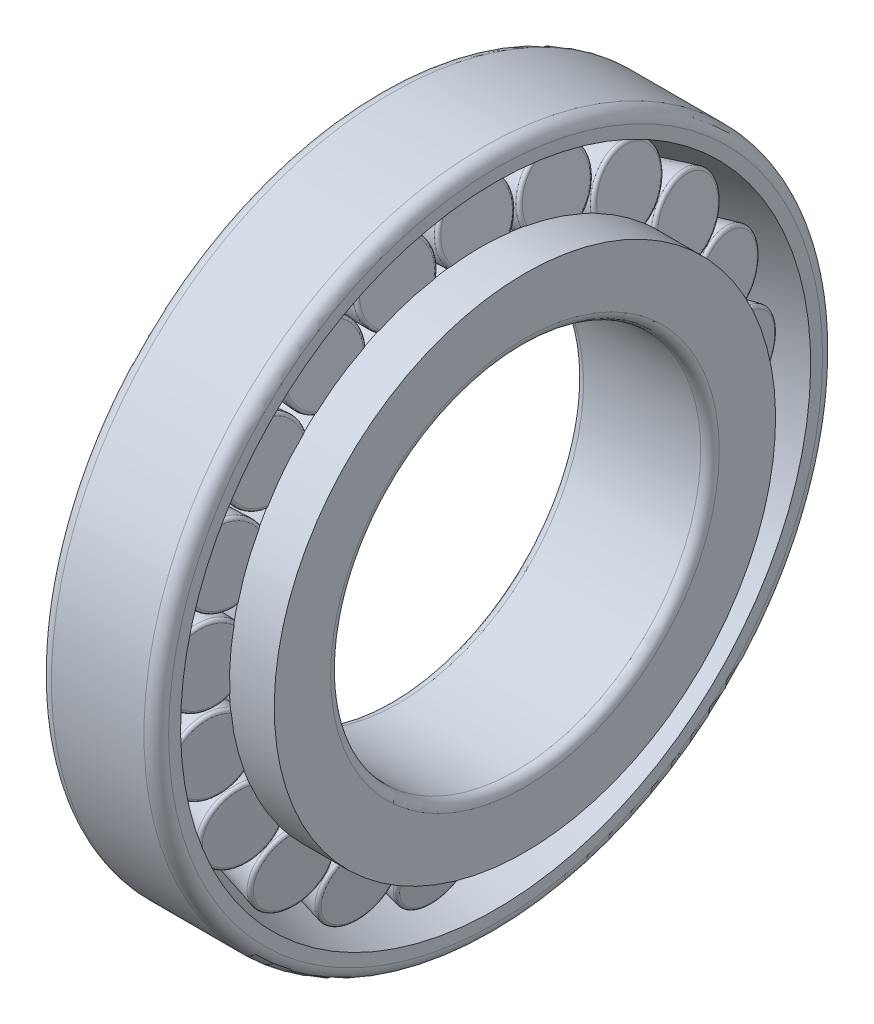
from build123d import *

# Parameters (mm, degrees)
CIRCULAR_PATTERN1_COUNT = 21


with BuildPart() as part:
    # Sketch1 → Revolve1 (revolve)
    with BuildSketch(Plane.XY):
        with BuildLine():
            Line((14.25, 40.629510659), (6.965132405, 40.629510659))
            Line((6.965132405, 40.629510659), (7.5, 37.629510659))
            Line((7.5, 37.629510659), (-4.744605679, 36.53476999))
            Line((-4.744605679, 36.53476999), (-5.012039477, 38.03476999))
            Line((-5.012039477, 38.03476999), (-7.75, 38.03476999))
            Line((-7.75, 38.03476999), (-7.75, 31.5))
            ThreePointArc((-7.75, 31.5), (-7.310660172, 30.439339828), (-6.25, 30))
            Line((-6.25, 30), (12.75, 30))
            ThreePointArc((12.75, 30), (13.810660172, 30.439339828), (14.25, 31.5))
            Line((14.25, 31.5), (14.25, 40.629510659))
        make_face()
    revolve(axis=Axis((14.25, 0, 0), (-1, 0, 0)))

    # Sketch2 → Revolve2 (revolve)
    with BuildSketch(Plane.XY):
        with BuildLine():
            Line((-5.673242352, 41.62942125), (6.422680954, 43.78599372))
            Line((6.422680954, 43.78599372), (7.42774649, 38.148717062))
            ThreePointArc((7.42774649, 38.148717062), (7.332763688, 37.757330854), (6.980034057, 37.562942832))
            Line((6.980034057, 37.562942832), (-4.304733142, 36.55401744))
            ThreePointArc((-4.304733142, 36.55401744), (-4.652884041, 36.654775976), (-4.841496329, 36.9642703))
            Line((-4.841496329, 36.9642703), (-5.673242352, 41.62942125))
        make_face()
    revolve2 = revolve(axis=Axis((-5.673242352, 41.62942125, 0), (0.9844756212878085, 0.17552136932574172, 0)))

    # Sketch3 → Revolve3 (revolve)
    with BuildSketch(Plane.XY):
        with BuildLine():
            Line((-9.5, 45.938), (9.5, 51.067795379))
            Line((9.5, 51.067795379), (9.5, 53))
            ThreePointArc((9.5, 53), (8.914213562, 54.414213562), (7.5, 55))
            Line((7.5, 55), (-7.5, 55))
            ThreePointArc((-7.5, 55), (-8.914213562, 54.414213562), (-9.5, 53))
            Line((-9.5, 53), (-9.5, 45.938))
        make_face()
    revolve(axis=Axis((14.25, 0, 0), (-1, 0, 0)))

    # Circular-Pattern1: Revolve2 ×21 about axis
    circular_pattern1_axis = Axis((0, 0, 0), (1, 0, 0))
    for i in range(1, CIRCULAR_PATTERN1_COUNT):
        add(revolve2.rotate(circular_pattern1_axis, i * 360 / CIRCULAR_PATTERN1_COUNT))


solid = part.part
